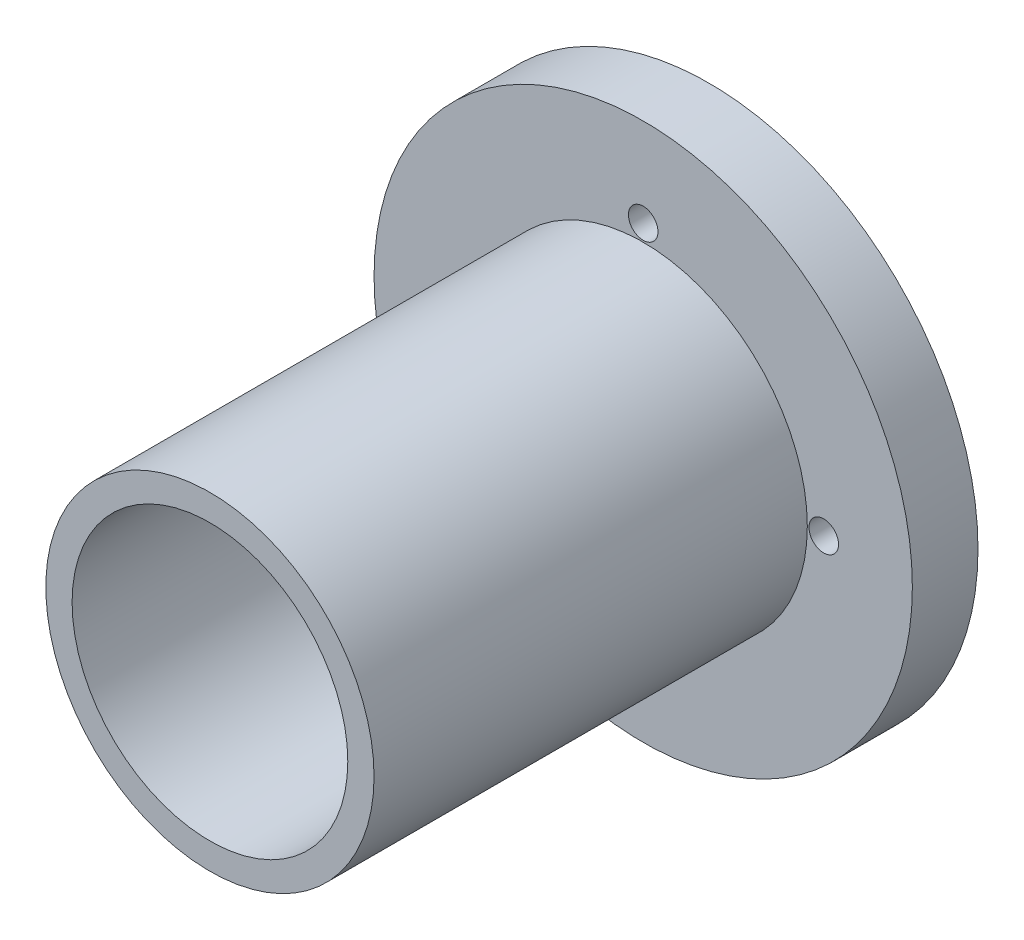
SolidWorks part; units mm, degrees
ref_plane "前视基准面" through (0, 0, 0) normal (0, 0, 1) x (1, 0, 0)
ref_plane "上视基准面" through (0, 0, 0) normal (0, 1, 0) x (1, 0, 0)
ref_plane "右视基准面" through (0, 0, 0) normal (1, 0, 0) x (0, 0, -1)
sketch "草图1" plane through (0, 0, 0) normal (0, 0, 1) x (1, 0, 0)
  circle A0 centre (0, 0) radius 21
  circle A1 centre (0, 0) radius 25
  dimension "D1" = 42
  dimension "D2" = 50
extrude "凸台-拉伸1" add sketch "草图1" along normal blind 66
sketch "草图2" plane through (0, 0, 0) normal (0, 0, -1) x (-1, 0, 0)
  circle A0 centre (0, 0) radius 41
  circle A1 centre (0, 0) radius 21 construction
  circle A2 centre (0, 0) radius 21
  dimension "D1" = 82
extrude "凸台-拉伸2" add sketch "草图2" along normal blind 10
sketch "草图3" plane through (0, 0, -10) normal (0, 0, -1) x (-1, 0, 0)
  circle A0 centre (0, 0) radius 27.5
  point P3 (0, -27.5)
  dimension "D1" = 55
hole_wizard "打孔尺寸(%根据)内六角圆柱头螺钉的类型1" positions "3D草图1" profile "草图4" counterbore size "M4" standard "GB" end condition up to next
sketch3d "3D草图1"
  point P0 (0, -27.5, -10)
sketch "草图4" plane through (0, -27.5, -10) normal (1, 0, 0) x (0, 1, 0)
  line L0 (0, 0) -> (0, 10.001)
  line L1 (0, 10.001) -> (2.25, 10.001)
  line L3 (2.25, 10.001) -> (2.25, 4.6)
  line L4 (2.25, 4.6) -> (4, 4.6)
  line L5 (4, 4.6) -> (4, 0)
  line L7 (4, 0) -> (0, 0)
  line L11 (0, -6.35) -> (0, 107.95) construction
  dimension "通孔孔直径" = 4.5
  dimension "通孔孔深度" = 10.001
  dimension "柱形沉头孔直径" = 8
  dimension "柱形沉头孔深度" = 4.6
pattern_circular "阵列(圆周)1" count 4 over 360 about axis through (0, 0, 0) along (0, 0, 1) of "打孔尺寸(%根据)内六角圆柱头螺钉的类型1"
